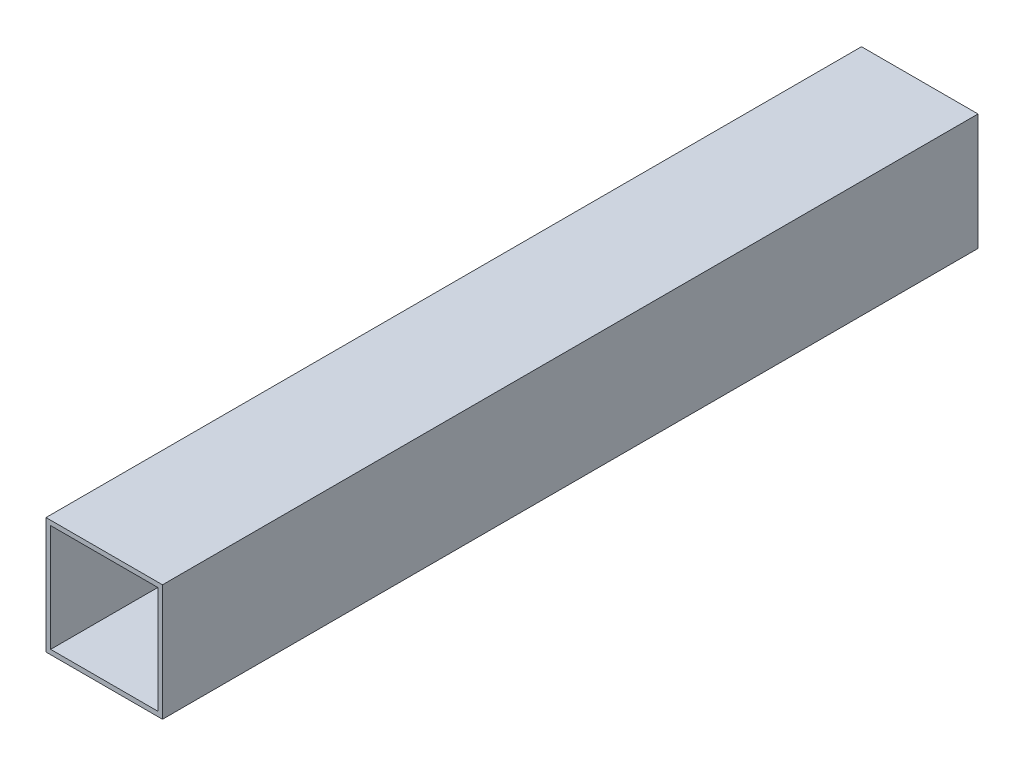
SolidWorks part; units mm, degrees
material "AISI 304"
ref_plane "Front Plane" through (0, 0, 0) normal (0, 0, 1) x (1, 0, 0)
ref_plane "Top Plane" through (0, 0, 0) normal (0, 1, 0) x (1, 0, 0)
ref_plane "Right Plane" through (0, 0, 0) normal (1, 0, 0) x (0, 0, -1)
sketch "Sketch1" plane through (0, 0, 0) normal (0, 0, 1) x (1, 0, 0)
  line L1 (-25, -25) -> (25, -25)
  line L2 (-25, -25) -> (-25, 25)
  line L3 (-25, 25) -> (25, 25)
  line L4 (25, -25) -> (25, 25)
  line L5 (-25, -25) -> (25, 25) construction
  line L6 (-25, 25) -> (25, -25) construction
  line L7 (-23, -23) -> (23, -23)
  line L8 (-23, -23) -> (-23, 23)
  line L9 (-23, 23) -> (23, 23)
  line L10 (23, -23) -> (23, 23)
  line L11 (-23, -23) -> (23, 23) construction
  line L12 (-23, 23) -> (23, -23) construction
  point P0 (0, 0)
  point P6 (0, 0)
  dimension "D1" = 50
  dimension "D2" = 50
  dimension "D3" = 46
  dimension "D4" = 46
extrude "Boss-Extrude1" add sketch "Sketch1" along normal blind 350
